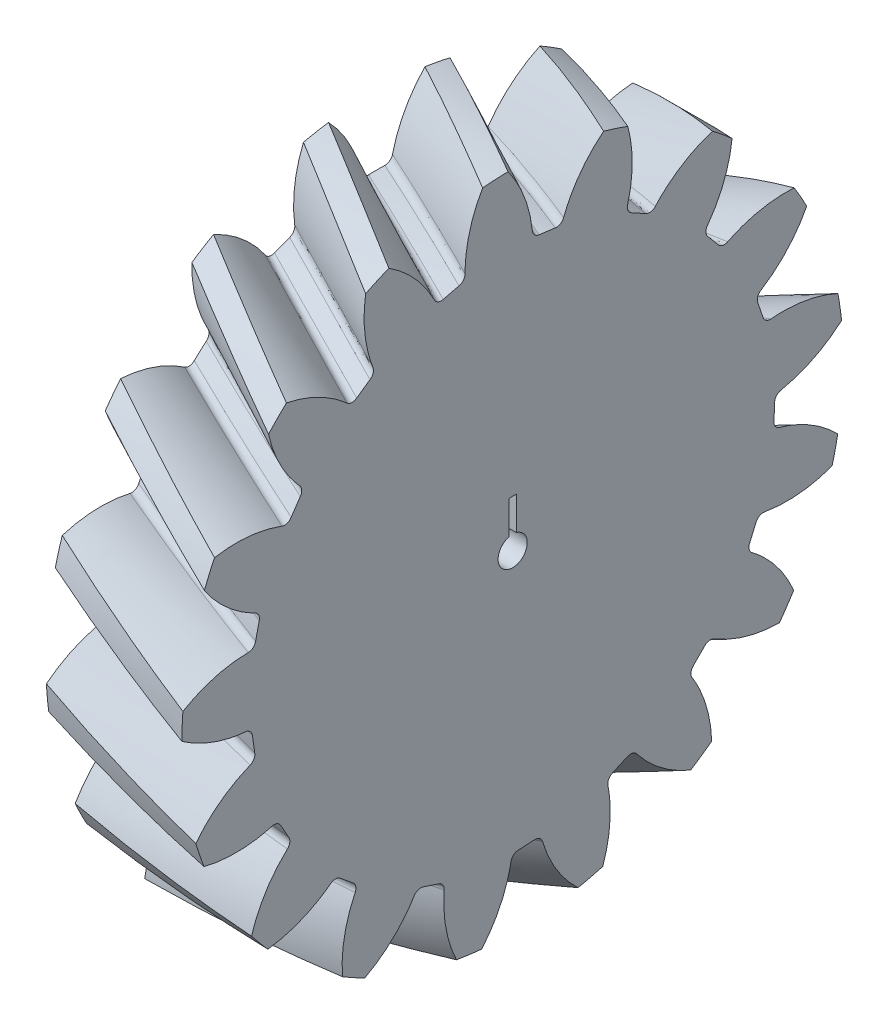
from build123d import *

# Parameters (mm, degrees)
BASPROSKE_W            = 44.45
BASPROSKE_H            = 108.149545762
TOOTHCUTRH_PITCH       = 1176.969464075
TOOTHCUTRH_HEIGHT      = 44.45
TOOTHCUTRH_RADIUS      = 108.149545762
TOOTHCUTRH_START_ANGLE = -90
TEETHCUTSRH_COUNT      = 17
TEETHCUTSRH_ANGLE      = 338.823529412
BORSKE_R               = 4.7625
BORE_DEPTH             = 130.0000025
KEYSKE_W               = 2.38252
KEYSKE_H               = 15.47876
KEYWAY_DEPTH           = 130.0000025


with BuildPart() as part:
    # BasProSke → Base-Revolve (revolve)
    with BuildSketch(Plane(origin=(0, 0, 0), x_dir=(1, 0, 0), z_dir=(0, 1, 0)), mode=Mode.PRIVATE) as base_revolve_sk:
        with Locations((22.225, 54.074772881)):
            Rectangle(BASPROSKE_W, BASPROSKE_H)
    revolve(base_revolve_sk.sketch.rotate(Axis((-10, 0, 0), (1, 0, 0)), 180), axis=Axis((-10, 0, 0), (1, 0, 0)))

    # ToothCutRH: sweep along a helix
    with BuildLine() as toothcutrh_path:
        add(Helix(TOOTHCUTRH_PITCH, TOOTHCUTRH_HEIGHT, TOOTHCUTRH_RADIUS, center=(0, 0, 0), direction=(1, 0, 0), mode=Mode.PRIVATE).rotate(Axis((0, 0, 0), (1, 0, 0)), TOOTHCUTRH_START_ANGLE))
    # TooCutSkeRH → ToothCutRH (sweep, cut)
    with BuildSketch(Plane(origin=(0, 0, 0), x_dir=(0, 0, -1), z_dir=(1, 0, 0))):
        with BuildLine():
            ThreePointArc((2.646465496, 85.608649736), (0, 85.649545762), (-2.646465496, 85.608649736))
            ThreePointArc((-2.646465496, 85.608649736), (-4.242297468, 86.121171594), (-5.156240123, 87.526186597))
            ThreePointArc((-5.156240123, 87.526186597), (-10.189401549, 99.734492405), (-18.726787404, 109.808641868))
            ThreePointArc((-18.726787404, 109.808641868), (0, 111.394032135), (18.726787404, 109.808641868))
            ThreePointArc((18.726787404, 109.808641868), (10.189401549, 99.734492405), (5.156240123, 87.526186597))
            ThreePointArc((5.156240123, 87.526186597), (4.242297468, 86.121171594), (2.646465496, 85.608649736))
        make_face()
    toothcutrh = sweep(path=toothcutrh_path.line, is_frenet=True, mode=Mode.SUBTRACT)

    # TeethCutsRH: ToothCutRH ×17 about axis
    teethcutsrh_axis = Axis((-10, 0, 0), (1, 0, 0))
    for i in range(1, TEETHCUTSRH_COUNT):
        add(toothcutrh.rotate(teethcutsrh_axis, i * TEETHCUTSRH_ANGLE / (TEETHCUTSRH_COUNT - 1)), mode=Mode.SUBTRACT)

    # BorSke → Bore (cut, symmetric)
    with BuildSketch(Plane(origin=(0, 0, 0), x_dir=(0, 0, -1), z_dir=(1, 0, 0))):
        with Locations(Location((0, 0, 0), (0, 0, 180))):
            Circle(BORSKE_R)
    extrude(amount=BORE_DEPTH, both=True, mode=Mode.SUBTRACT)

    # KeySke → Keyway (cut, symmetric)
    with BuildSketch(Plane(origin=(0, 0, 0), x_dir=(0, 0, -1), z_dir=(1, 0, 0))):
        with Locations((0, 7.73938)):
            Rectangle(KEYSKE_W, KEYSKE_H)
    extrude(amount=KEYWAY_DEPTH, both=True, mode=Mode.SUBTRACT)


solid = part.part
